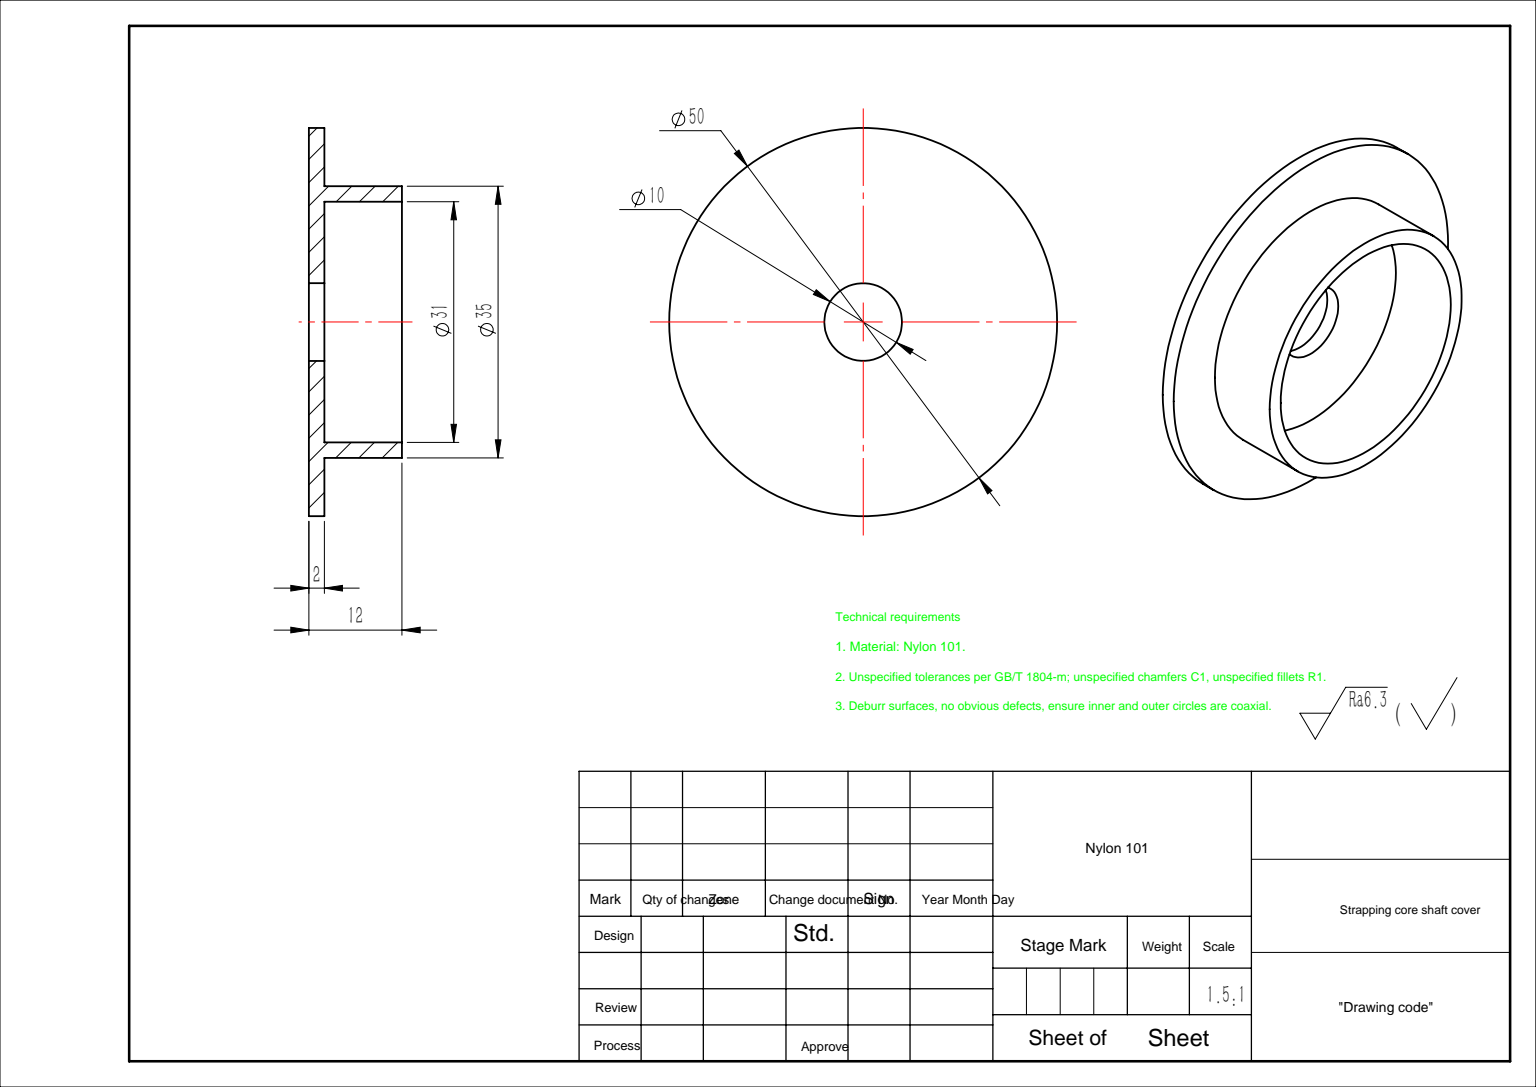
from build123d import *


with BuildPart() as part:
    # 草图1 → 旋转1 (revolve)
    with BuildSketch(Plane.XY, mode=Mode.PRIVATE) as revolve_1_sk:
        Polygon((0, 25), (2, 25), (2, 17.5), (12, 17.5), (12, 15.5), (2, 15.5), (2, 5), (0, 5), align=None)
    revolve(revolve_1_sk.sketch.rotate(Axis((0, 0, 0), (1, 0, 0)), 90), axis=Axis((0, 0, 0), (1, 0, 0)))


solid = part.part
